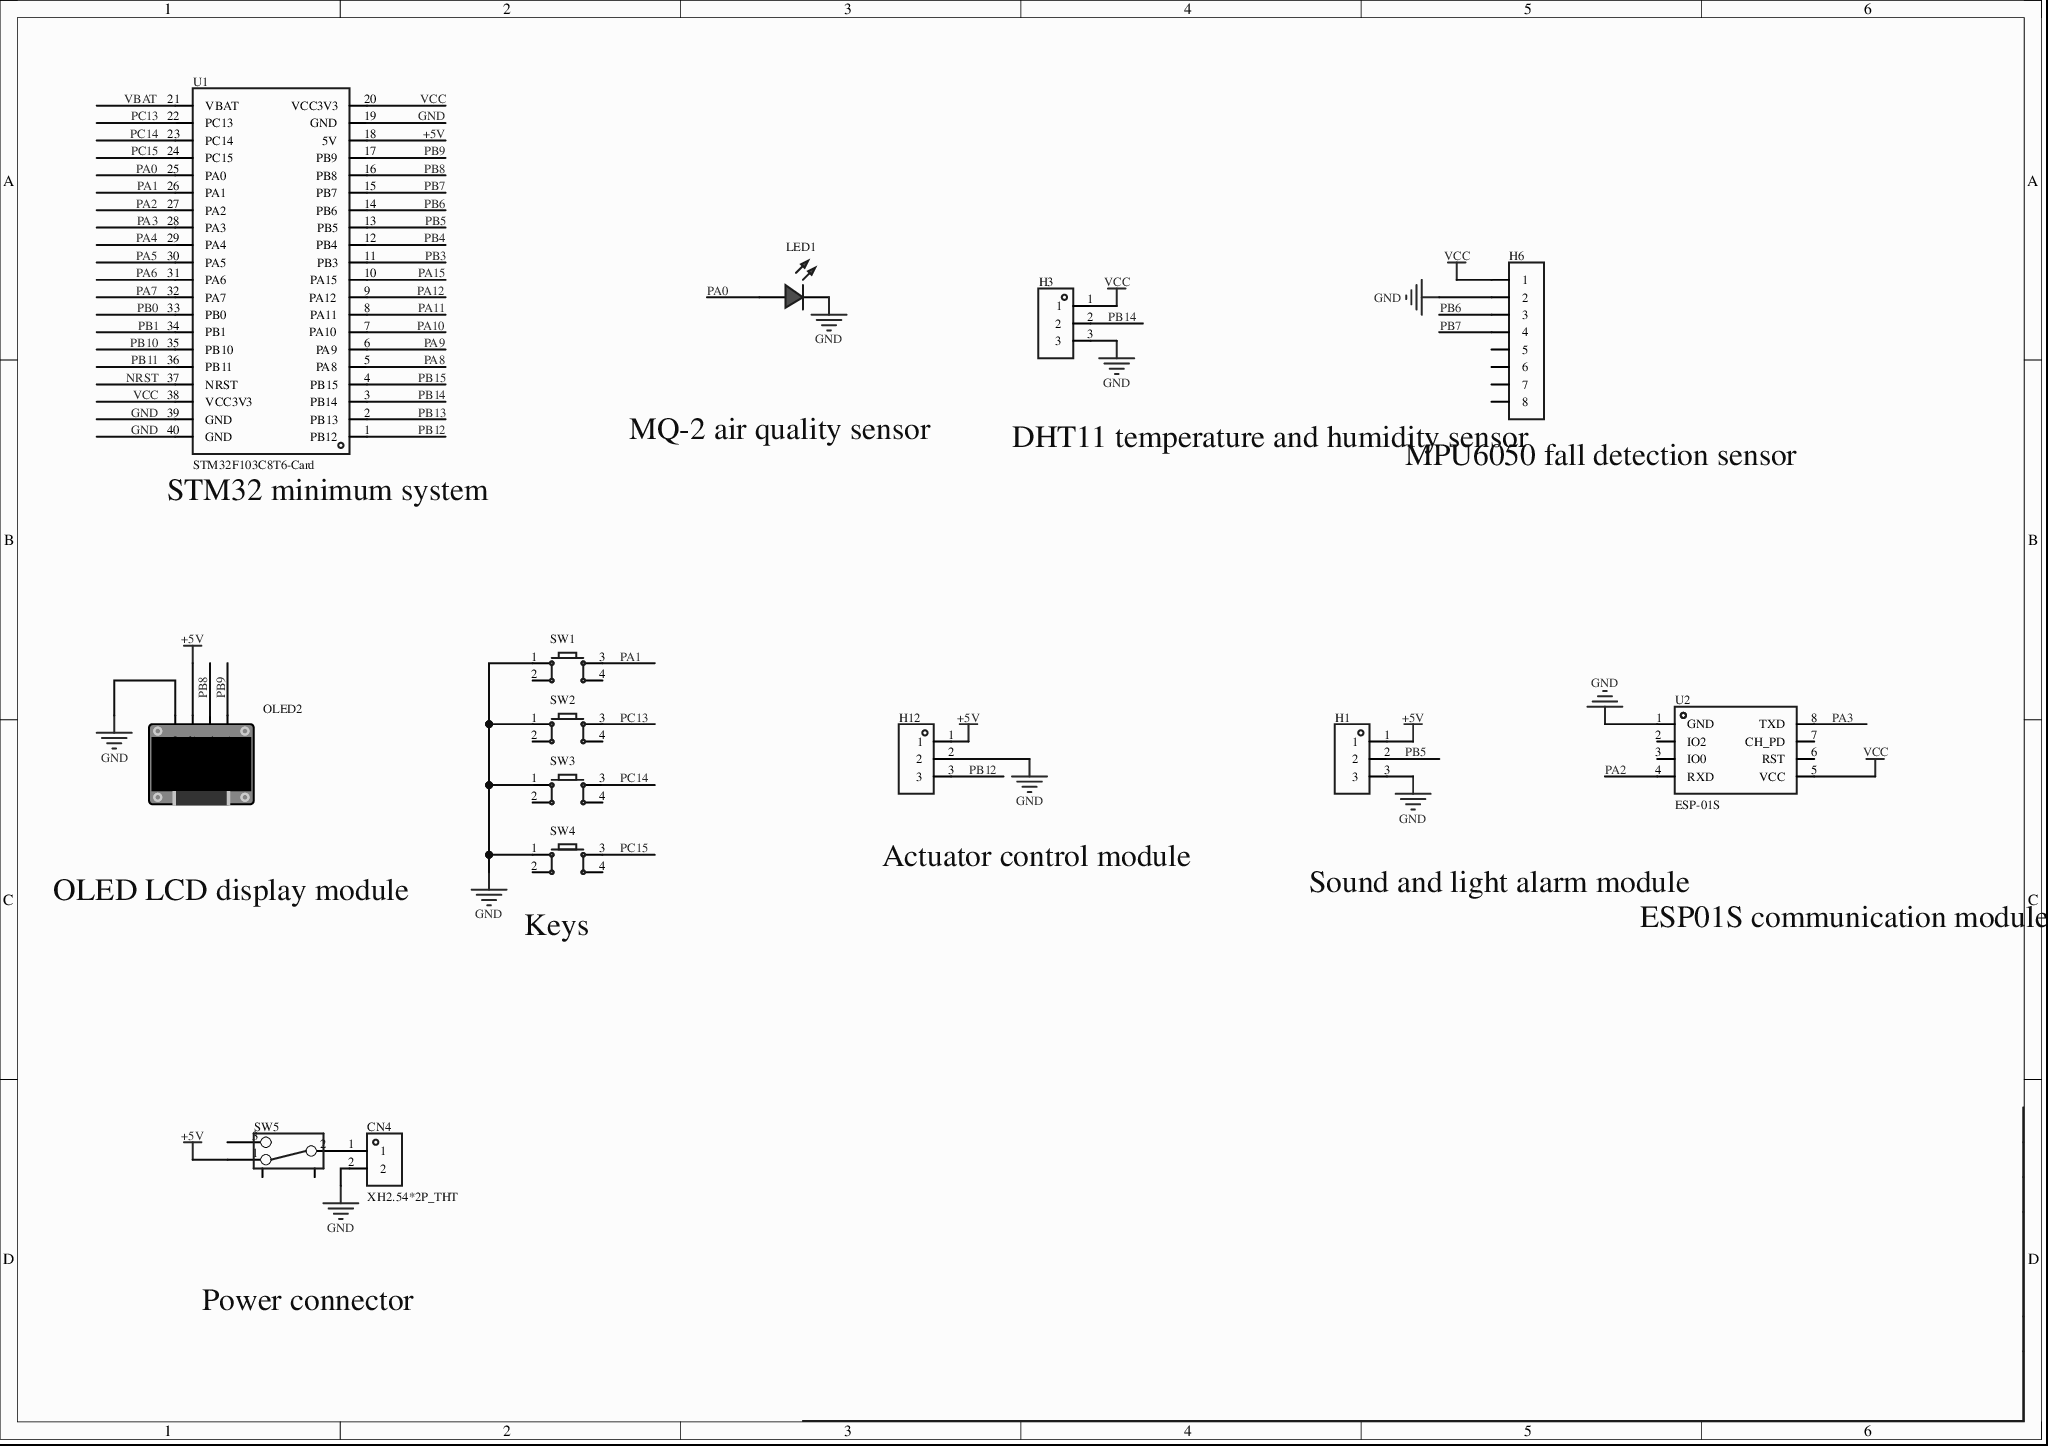
[diagram p0: MISC51555-3.schdoc]
# Altium project MISC51555-2.PrjPcb
1 sheet, 14 parts. Net scope: global (net labels, ports and power ports of the same name join across sheets).
Board file: MISC51555.pcbdoc

## Sheet MISC51555-3.schdoc
size 297 x 209 mm; Version: V1.0; @Project Name: MISC51555; @Page Count: 1; @Update Date: 2026-04-28; @Create Date: 2026-04-28; @Schematic Name: MISC51555; @Page No: 1; @Create Time: 23:22:16; @Update Time: 17:32:40; @Board Name: MISC51555

### Parts
CN4  XH2.54*2P_THT  [CONN-TH_2P-P2.50-XH2.54-2P]
H1  (no value)  [HDR-TH_3P-P2.54-V-F]
H3  (no value)  [HDR-TH_3P-P2.54-V-F]
H6  (no value)  [HDR-TH_8P-P2.54-V-F-1]
H12  (no value)  [HDR-TH_3P-P2.54-V-F]
LED1  (no value)  [LED_TH-3mm]
OLED2  (no value)  [0.96OLED_4P]
SW1  (no value)  [SW-TH_4P-L6.0-W6.0-P4.50-LS6.5]
SW2  (no value)  [SW-TH_4P-L6.0-W6.0-P4.50-LS6.5]
SW3  (no value)  [SW-TH_4P-L6.0-W6.0-P4.50-LS6.5]
SW4  (no value)  [SW-TH_4P-L6.0-W6.0-P4.50-LS6.5]
SW5  (no value)  [拨动开关]
U1  STM32F103C8T6-Card  [CONN-TH_L53.3-W22.9_STM32F103C8T6-CARD]
U2  ESP-01S  [WIFIM-TH_ESP-01S]

### Nets
+5V: H1.1 H12.1 OLED2.2(VCC) SW5.1 U1.18(5V)
GND: CN4.2 H1.3 H3.3 H6.2 H12.2 LED1.2(A) OLED2.1(GND) SW1.1 SW2.1 SW3.1 SW4.1 U1.19(GND) U1.39(GND) U1.40(GND) U2.1(GND)
VCC: H3.1 H6.1 U1.20(VCC3V3) U1.38(VCC3V3) U2.5(VCC)
NRST: U1.37(NRST)
PA0: LED1.1(C) U1.25(PA0)
PA1: SW1.3 U1.26(PA1)
PA2: U1.27(PA2) U2.4(RXD)
PA3: U1.28(PA3) U2.8(TXD)
PA4: U1.29(PA4)
PA5: U1.30(PA5)
PA6: U1.31(PA6)
PA7: U1.32(PA7)
PA8: U1.5(PA8)
PA9: U1.6(PA9)
PA10: U1.7(PA10)
PA11: U1.8(PA11)
PA12: U1.9(PA12)
PA15: U1.10(PA15)
PB0: U1.33(PB0)
PB1: U1.34(PB1)
PB3: U1.11(PB3)
PB4: U1.12(PB4)
PB5: H1.2 U1.13(PB5)
PB6: H6.3 U1.14(PB6)
PB7: H6.4 U1.15(PB7)
PB8: OLED2.3(SCL) U1.16(PB8)
PB9: OLED2.4(SDA) U1.17(PB9)
PB10: U1.35(PB10)
PB11: U1.36(PB11)
PB12: H12.3 U1.1(PB12)
PB13: U1.2(PB13)
PB14: H3.2 U1.3(PB14)
PB15: U1.4(PB15)
PC13: SW2.3 U1.22(PC13)
PC14: SW3.3 U1.23(PC14)
PC15: SW4.3 U1.24(PC15)
VBAT: U1.21(VBAT)
NetCN4_1: CN4.1 SW5.2

Not connected (* = marked no-connect by the designer): H6 5 6 7 8; SW1 2 4; SW2 2 4; SW3 2 4; SW4 2 4; SW5 3 4 5; U2 2(IO2)* 3(IO0)* 6(RST)* 7(CH_PD)*

### Notes on the sheet
- (near U1) STM32 minimum system
- MQ-2 air quality sensor
- (near H6) DHT11 temperature and humidity sensor
- (near H6) MPU6050 fall detection sensor
- (near H12) Actuator control module
- OLED LCD display module
- (near SW4) Keys
- Sound and light alarm module
- ESP01S communication module
- Power connector

### Library data of the parts
CN4 = XH2.54*2P_直插: 3D Model: 325c595e30db4df8abe76612dd40b0fa0819f05c4eef4c71ace90d822a990e87; 3D Model Transform: 295.275,228.346,0,180,0,0,-0.002,-20.079,-137.795; AddInBom: yes; Device: XH2.54*2P_THT; Symbol: XH2.54*2P_THT; LCSC Part Name: XH2.54*2P_直插; Supplier Part: C9900008615; Manufacturer Part: XH2.54*2P_直插; Supplier Footprint: XH2.54_2P; JLCPCB Part Class: Extended Part; Supplier: LCSC; FootprintName: CONN-TH_2P-P2.50-XH2.54-2P; ConvertToPcb: yes; ModelName: CONN-TH_2P-P2.50-XH2.54-2P
H1 H3 H12 = HDR-F_2.54_1x3P: Symbol: PM254V-11-03-H85; 3D Model: f3b3cc5aae9641bf9e56fc160cef875b; 3D Model Transform: 299.9994,100,0,0,0,0,0,0,-118.11; ConvertToPcb: yes; ModelName: HDR2.54-F-LI-1X3P; Device: HDR-F_2.54_1x3P; Supplier Part: C541850; Supplier Footprint: 插件; FootprintName: HDR-TH_3P-P2.54-V-F; AddInBom: yes
H6 = HDR-F_2.54_1x8P: Symbol: Header-Female-2.54_1x8; AddInBom: yes; ModelId: 0f7e4d9227ef4fa08d5469c22cc70cdb; ModelName: HDR-F-2.54_1x8; ModelTransform: 799.99844,100,0,0,0,0,0,0,-118.11; Device: HDR-F_2.54_1x8P; ConvertToPcb: yes; FootprintName: HDR-TH_8P-P2.54-V-F-1; SupplierPart: C27438; Supplier Footprint: 插件
LED1 = LED_TH-R_3mm: ConvertToPcb: yes; ModelId: a497c992633541038a38947cdc58012f0819f05c4eef4c71ace90d822a990e87; ModelName: LED-TH-3mm_R; ModelTransform: 141.274,153.327,0,0,0,0,-5.984,0,-137.795; Symbol: LED_TH-R; Device: LED_TH-R_3mm; AddInBom: yes; FootprintName: LED_TH-3mm; Supplier Footprint: 插件
OLED2 = 0.96OLED模块_4P: Symbol: 0.96OLED module_4P; 3D Model: 79c000fdb68d45a296c2e9bedf4f9055; 3D Model Transform: 1393.69792,1318.895,0,0,0,0,0,-560.079,-137.795; ConvertToPcb: yes; Device: 0.96OLED module_4P; Supplier Footprint: 插件; AddInBom: yes; FootprintName: 0.96OLED_4P; ModelName: 0.96OLED_4P
SW1-SW4 = Key_TH_6x6x6: 触点电流:50mA;额定电压(DC):12V;绝缘电阻:100MΩ;电路结构:单刀单掷;安装方式:直插;按钮形状:圆形按钮;按钮/盖帽颜色:黑色;作用力:260gf@±30gf;工作温度:-25℃~+70℃;引脚样式:PC引脚;开关长度:6mm;开关宽度:6mm;开关高度:6mm;带支架:否;; Symbol: Tactile switch; AddInBom: yes; ModelId: 20eee248bc684ccd8cbdbb1d0d91ec6f0819f05c4eef4c71ace90d822a990e87; ModelName: SW-TH_4P-L6.0-W6.0-H5.0-LS6.5-P4.50; ModelTransform: 236.22,323.03,0,90,0,0,0,0,-137.795; Device: Key_TH_6x6x6; FootprintName: SW-TH_4P-L6.0-W6.0-P4.50-LS6.5; ConvertToPcb: yes; Supplier Footprint: 插件
SW5 = 拨动开关_正: Device: Toggle switch_pos; Symbol: Toggle switch; 3D Model: 4321fe59a4074cbfb4989553f297c68f0819f05c4eef4c71ace90d822a990e87; 3D Model Transform: 370.09,208.7,472.35,0,0,0,0,0,-110; ConvertToPcb: yes; ModelName: SW-TH_SS-12D02-VG4; Supplier Footprint: 插件; FootprintName: Toggle switch; AddInBom: yes
U1 = STM32F103C8T6-Card: AddInBom: yes; Device: STM32F103C8T6-Card; Symbol: STM32F103C8T6-CARD; FootprintName: CONN-TH_L53.3-W22.9_STM32F103C8T6-CARD; LCSC Part Name: STM32F103C8T6-Card; SupplierPart: C9900077949; ManufacturerPart: STM32F103C8T6-Card; Supplier Footprint: 插件; Supplier: LCSC; ConvertToPcb: yes
U2 = ESP-01S_C111009: 3D Model: eb7175da78ae48b3b1568cfe3027405f0819f05c4eef4c71ace90d822a990e87; 3D Model Transform: 582.676,976.37608,0,0,0,0,0,388.346,-118.11; AddInBom: yes; Symbol: ESP-01S; Device: ESP-01S_C111009; LCSC Part Name: ESP-01S; Supplier Part: C111009; Manufacturer Part: ESP-01S; Supplier Footprint: -; JLCPCB Part Class: Extended Part; Supplier: LCSC; ConvertToPcb: yes; FootprintName: WIFIM-TH_ESP-01S; ModelName: WIFIM-TH_ESP-01S